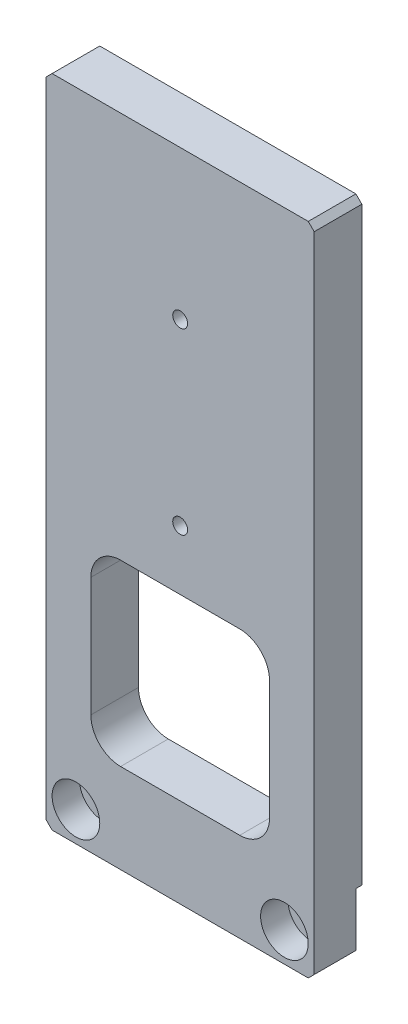
SolidWorks part; units mm, degrees
material "A6061"
ref_plane "Front Plane" through (0, 0, 0) normal (0, 0, 1) x (1, 0, 0)
ref_plane "Top Plane" through (0, 0, 0) normal (0, 1, 0) x (1, 0, 0)
ref_plane "Right Plane" through (0, 0, 0) normal (1, 0, 0) x (0, 0, -1)
sketch "Sketch1" plane through (0, 0, 0) normal (0, 0, 1) x (1, 0, 0)
  line L1 (-22.5, -55) -> (22.5, -55)
  line L2 (-22.5, -55) -> (-22.5, 55)
  line L3 (-22.5, 55) -> (22.5, 55)
  line L4 (22.5, -55) -> (22.5, 55)
  line L5 (-22.5, -55) -> (22.5, 55) construction
  line L6 (-22.5, 55) -> (22.5, -55) construction
  point P0 (0, 0)
  dimension "D1" = 45
  dimension "D2" = 110
extrude "Boss-Extrude1" add sketch "Sketch1" along normal mid plane 8
hole_wizard "Hole size (% based on socket head cap screw type)1" positions "Sketch3" profile "Sketch2" counterbore size "M4" standard "GB"
sketch "Sketch3" plane through (0, 0, 4) normal (0, 0, 1) x (1, 0, 0)
  line L0 (0, 0) -> (0, -84.2182) construction
  line L4 (-22.5, -55) -> (22.5, -55) construction
  point P0 (-17.5, -50)
  point P2 (17.5, -50)
  dimension "D1" = 35
  dimension "D2" = 5
sketch "Sketch2" plane through (-17.5, -50, 4) normal (1, 0, 0) x (0, -1, 0)
  line L0 (0, 0) -> (0, 13.7519)
  line L1 (0, 13.7519) -> (2.25, 12.4)
  line L2 (2.25, 12.4) -> (2.25, 4.6)
  line L3 (2.25, 4.6) -> (4, 4.6)
  line L4 (4, 4.6) -> (4, 0)
  line L5 (4, 0) -> (0, 0)
  line L10 (0, 13.7519) -> (-2.25, 12.4) construction
  line L11 (0, -6.35) -> (0, 107.95) construction
  dimension "孔直径" = 4.5
  dimension "孔深度" = 12.4
  dimension "柱形沉头孔直径" = 8
  dimension "柱形沉头孔深度" = 4.6
  dimension "导头角度" = 118
sketch "Sketch4" plane through (22.5, 0, 0) normal (1, 0, 0) x (0, 0, -1)
  line L1 (4, -55) -> (3, -55)
  line L2 (4, -55) -> (4, -45)
  line L3 (4, -45) -> (3, -45)
  line L4 (3, -55) -> (3, -45)
  dimension "D1" = 1
  dimension "D2" = 10
extrude "Cut-Extrude1" cut sketch "Sketch4" against normal through all
hole_wizard "M3 Tapped Hole1" positions "Sketch6" profile "Sketch5" tap size "M3" standard "ISO" end condition through all
sketch "Sketch6" plane through (0, 0, 4) normal (0, 0, 1) x (1, 0, 0)
  line L0 (-22.5, -55) -> (22.5, -55) construction
  point P0 (0, 30)
  point P2 (0, 0)
  dimension "D1" = 30
  dimension "D2" = 55
sketch "Sketch5" plane through (0, 30, 4) normal (1, 0, 0) x (0, -1, 0)
  line L0 (0, 0) -> (0, 8)
  line L1 (0, 8) -> (1.25, 8)
  line L2 (1.25, 8) -> (1.25, 0)
  line L5 (1.25, 0) -> (0, 0)
  line L11 (0, -6.35) -> (0, 107.95) construction
  dimension "通孔螺纹孔钻头直径" = 2.5
  dimension "通孔螺纹孔钻头深度" = 8
cosmetic thread "Hole thread1" parameters "D2"=3
cosmetic thread "Hole thread2" parameters "D2"=3
chamfer "Chamfer1" distance 1 angle 45 4 edges at (-22.5, 55, 0) (22.5, 55, 0) (-22.5, -55, 0.5) (22.5, -55, 0.5)
sketch "Sketch7" plane through (0, 0, 4) normal (0, 0, 1) x (1, 0, 0)
  line L0 (0, -55) -> (0, 10.3108) construction
  line L1 (10, -10) -> (-10, -10)
  line L2 (15, -15) -> (15, -35)
  line L3 (10, -40) -> (-10, -40)
  line L4 (-15, -15) -> (-15, -35)
  line L5 (-21.5, -55) -> (21.5, -55) construction
  arc A0 (10, -10) -> (15, -15) centre (10, -15) cw
  arc A1 (-10, -10) -> (-15, -15) centre (-10, -15) ccw
  arc A2 (-10, -40) -> (-15, -35) centre (-10, -35) cw
  arc A3 (15, -35) -> (10, -40) centre (10, -35) cw
  point P13 (-15, -10)
  point P16 (-15, -40)
  point P19 (15, -40)
  dimension "D4" = 5
  dimension "D1" = 30
  dimension "D2" = 30
  dimension "D3" = 15
extrude "Cut-Extrude2" cut sketch "Sketch7" against normal through all
